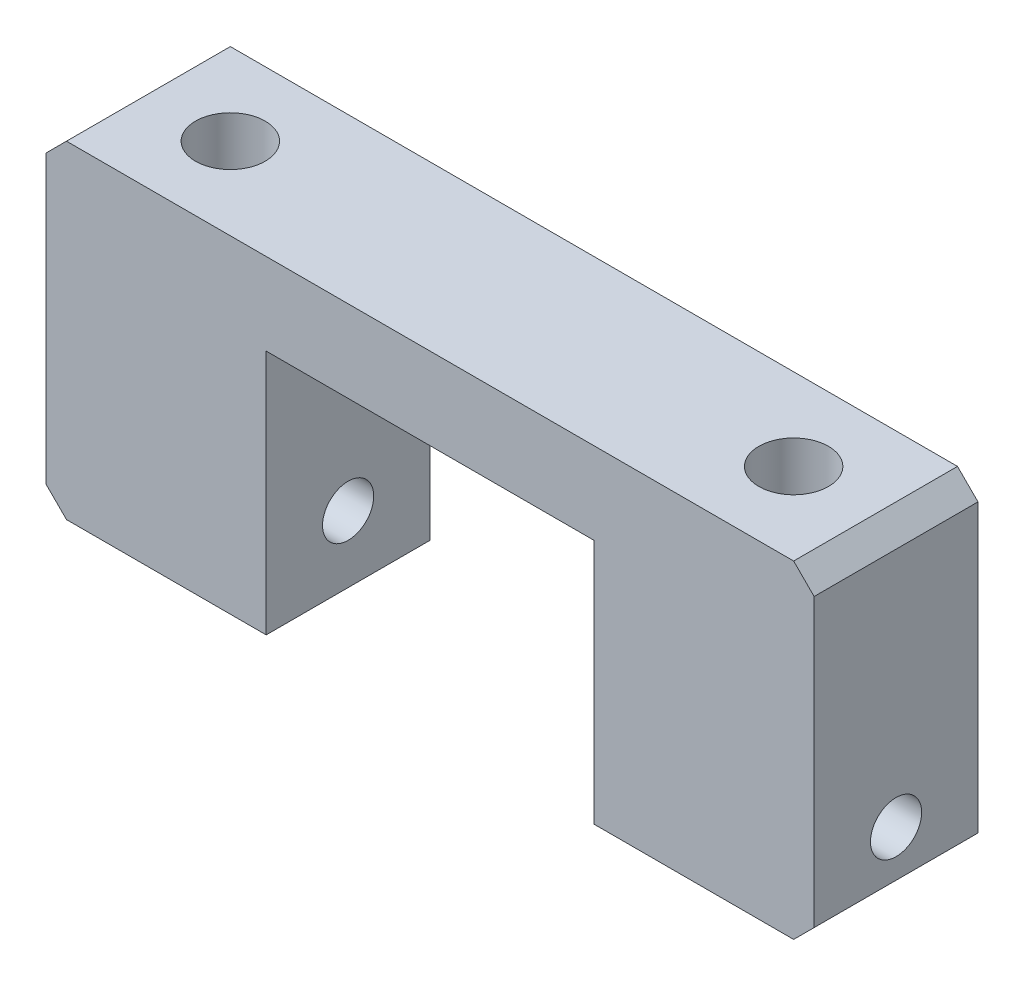
SolidWorks part; units mm, degrees
ref_plane "前视基准面" through (0, 0, 0) normal (0, 0, 1) x (1, 0, 0)
ref_plane "上视基准面" through (0, 0, 0) normal (0, 1, 0) x (1, 0, 0)
ref_plane "右视基准面" through (0, 0, 0) normal (1, 0, 0) x (0, 0, -1)
sketch "草图1" plane through (0, 0, 0) normal (0, 0, 1) x (1, 0, 0)
  line L0 (0, 16) -> (0, 0) construction
  line L1 (-37.5, 16) -> (37.5, 16)
  line L2 (-37.5, 16) -> (-37.5, -16)
  line L3 (-37.5, -16) -> (37.5, -16)
  line L4 (37.5, 16) -> (37.5, -16)
  line L5 (0, 0) -> (37.5, 0) construction
  dimension "D1" = 75
  dimension "D2" = 32
extrude "凸台-拉伸1" add sketch "草图1" along normal mid plane 16
sketch "草图3" plane through (0, 0, 8) normal (0, 0, 1) x (1, 0, 0)
  line L0 (-37.5, -16) -> (37.5, -16) construction
  line L1 (-16, -16) -> (16, -16)
  line L2 (-16, -16) -> (-16, 8)
  line L3 (-16, 8) -> (16, 8)
  line L4 (16, -16) -> (16, 8)
  line L5 (0, 24) -> (0, 0) construction
  line L6 (0, 0) -> (44.4811, 0) construction
  line L7 (37.5, 16) -> (-37.5, 16) construction
  dimension "D1" = 32
  dimension "D2" = 8
extrude "切除-拉伸1" cut sketch "草图3" against normal through all
hole_wizard "M6 螺纹孔1" positions "草图7" profile "草图6" tap size "M6" standard "Iso" end condition through all
sketch "草图7" plane through (37.5, 0, 0) normal (1, 0, 0) x (0, 0, -1)
  line L0 (0, 0) -> (0, -16.1416) construction
  line L3 (-8, 16) -> (8, 16) construction
  point P0 (0, -9.5)
  dimension "D1" = 25.5
sketch "草图6" plane through (37.5, -9.5, 0) normal (0, 1, 0) x (0, 0, -1)
  line L0 (0, 0) -> (0, 75)
  line L1 (0, 75) -> (2.5, 75)
  line L2 (2.5, 75) -> (2.5, 0)
  line L5 (2.5, 0) -> (0, 0)
  line L11 (0, -6.35) -> (0, 107.95) construction
  dimension "通孔螺纹孔钻头直径" = 5
  dimension "通孔螺纹孔钻头深度" = 75
cosmetic thread "孔螺蚊线4" parameters "D2"=6
chamfer "倒角1" distance 2 angle 45 2 edges at (-37.5, 16, 0) (37.5, 16, 0)
hole_wizard "M8 螺纹孔1" positions "草图9" profile "草图8" tap size "M8" standard "ISO"
sketch "草图9" plane through (0, 16, 0) normal (0, 1, 0) x (1, 0, 0)
  line L0 (0, 13.8881) -> (0, 0) construction
  line L1 (0, 0) -> (44.4811, 0) construction
  point P0 (-27.5, 0)
  point P2 (27.5, 0)
  dimension "D1" = 55
sketch "草图8" plane through (-27.5, 16, 0) normal (1, 0, 0) x (0, 0, 1)
  line L0 (0, 0) -> (0, 21.7929)
  line L1 (0, 21.7929) -> (3.4, 19.75)
  line L2 (3.4, 19.75) -> (3.4, 0)
  line L5 (3.4, 0) -> (0, 0)
  line L10 (0, 21.7929) -> (-3.4, 19.75) construction
  line L11 (0, -6.35) -> (0, 107.95) construction
  dimension "螺纹孔钻头直径" = 6.8
  dimension "螺纹孔钻头深度" = 19.75
  dimension "导头角度" = 118
cosmetic thread "孔螺蚊线2" parameters "D1"=16, "D2"=8
cosmetic thread "孔螺蚊线3" parameters "D1"=16, "D2"=8
chamfer "倒角2" distance 2 angle 45 2 edges at (37.5, -16, 0) (-37.5, -16, 0)
